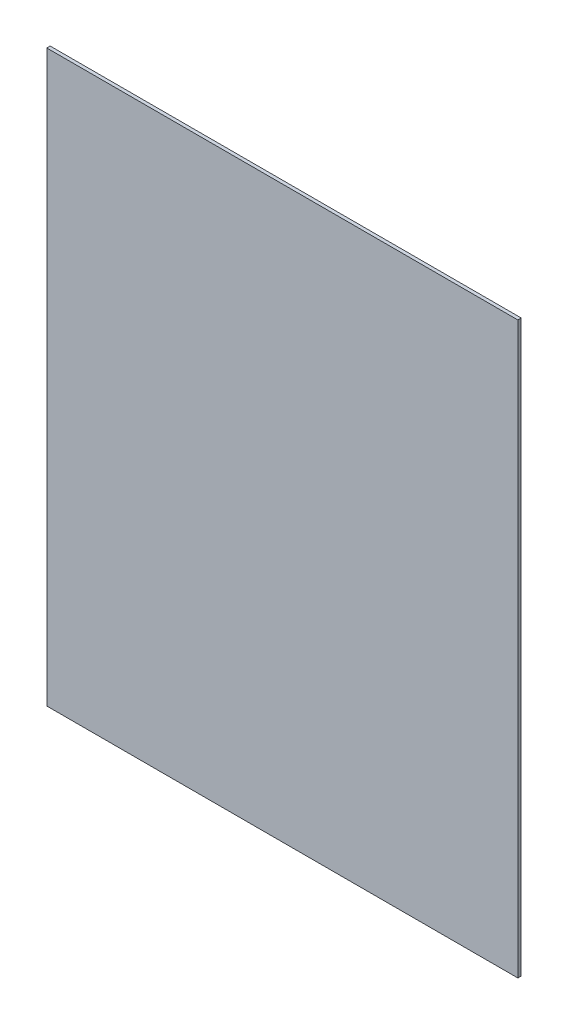
SolidWorks part; units mm, degrees
material "PMMA(有机玻璃)"
ref_plane "前视" through (0, 0, 0) normal (0, 0, 1) x (1, 0, 0)
ref_plane "上视" through (0, 0, 0) normal (0, 1, 0) x (1, 0, 0)
ref_plane "右视" through (0, 0, 0) normal (1, 0, 0) x (0, 0, -1)
sketch "草图1" plane through (0, 0, 0) normal (0, 0, 1) x (1, 0, 0)
  line L1 (-348, 421) -> (348, 421)
  line L2 (-348, 421) -> (-348, -421)
  line L3 (-348, -421) -> (348, -421)
  line L4 (348, 421) -> (348, -421)
  line L5 (-348, 421) -> (348, -421) construction
  line L6 (-348, -421) -> (348, 421) construction
  point P0 (0, 0)
  dimension "D1" = 842
  dimension "D2" = 696
extrude "凸台-拉伸1" add sketch "草图1" along normal blind 5
hole_wizard "M5 间隙孔1" positions "草图3" profile "草图2" hole size "M5" standard "GB"
sketch "草图3" plane through (0, 0, 5) normal (0, 0, 1) x (1, 0, 0)
  line L0 (-427.5, 273) -> (-427.5, -273) construction
  line L1 (-427.5, -273) -> (427.5, -273) construction
  line L2 (0, 273) -> (0, -273) construction
  line L3 (427.5, 273) -> (-427.5, 273) construction
  line L5 (-427.5, 0) -> (427.5, 0) construction
  line L6 (427.5, -273) -> (427.5, 273) construction
  point P0 (-375, -261)
  point P46 (415.5, 250)
  point P48 (-415.5, 250)
  point P58 (-125, -261)
  point P59 (125, -261)
  point P61 (-125, 261)
  point P62 (125, 261)
  point P64 (-375, 261)
  point P88 (375, -261)
  point P89 (375, 261)
  point P108 (415.5, 0)
  point P109 (-415.5, 0)
  point P110 (415.5, -250)
  point P111 (-415.5, -250)
  dimension "D1" = 12
  dimension "D2" = 12
  dimension "D5" = 3
  dimension "D3" = 12
  dimension "D6" = 4
  dimension "D4" = 2
sketch "草图2" plane through (-375, -261, 5) normal (1, 0, 0) x (0, -1, 0)
  line L0 (0, 0) -> (0, 5)
  line L1 (0, 5) -> (2.75, 5)
  line L2 (2.75, 5) -> (2.75, 0)
  line L5 (2.75, 0) -> (0, 0)
  line L11 (0, -6.35) -> (0, 107.95) construction
  dimension "通孔孔直径" = 5.5
  dimension "通孔孔深度" = 5
